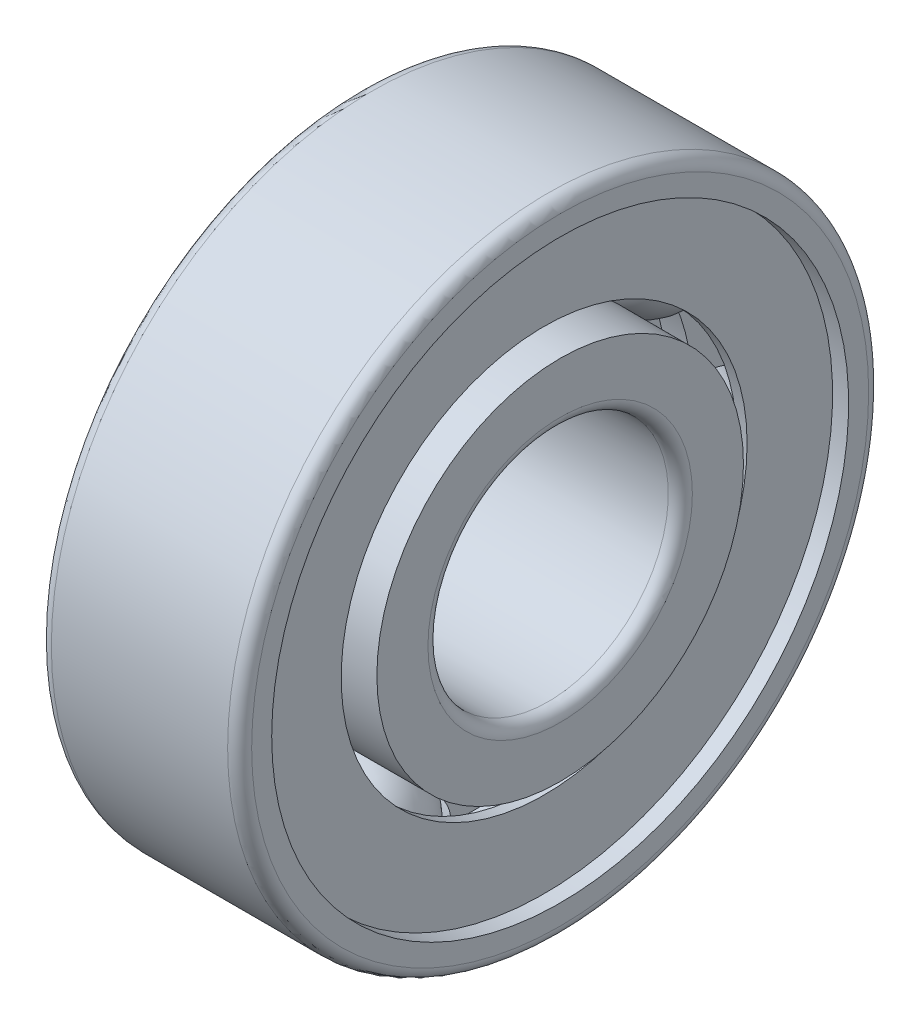
from build123d import *
from build123d.topology import SkipClean

# Parameters (mm, degrees)
SKETCH2_W          = 1.30966
SKETCH2_H          = 1.637075
CIRPATTERN1_COUNT  = 7
SKETCH4_W          = 6.5483
SKETCH4_H          = 3.27415
SKETCH5_W          = 6.5483
SKETCH5_H          = 3.27415
CIRPATTERN2_COUNT  = 7
SKETCH10_W         = 0.535202389
SKETCH10_H         = 3.867755
SKETCH11_R         = 16
CUT_EXTRUDE1_DEPTH = 10


with BuildPart() as part:
    # Sketch2 → Base-Revolve (revolve)
    with BuildSketch(Plane.XY, mode=Mode.PRIVATE) as base_revolve_sk:
        with Locations((0, 11.775)):
            Rectangle(SKETCH2_W, SKETCH2_H)
    revolve(base_revolve_sk.sketch.rotate(Axis((-12.420610377, 0, 0), (1, 0, 0)), 90), axis=Axis((-12.420610377, 0, 0), (1, 0, 0)))

    # Sketch3 → Boss-Revolve1 (revolve)
    with BuildSketch(Plane.XY):
        with BuildLine():
            Line((-3.27415, 11.775), (3.27415, 11.775))
            ThreePointArc((3.27415, 11.775), (0, 8.50085), (-3.27415, 11.775))
        make_face()
    boss_revolve1 = revolve(axis=Axis((-5.568093779, 11.775, 0), (1, 0, 0)))

    # CirPattern1: Boss-Revolve1 ×7 about axis
    cirpattern1_axis = Axis((0, 0, 0), (1, 0, 0))
    for i in range(1, CIRPATTERN1_COUNT):
        add(boss_revolve1.rotate(cirpattern1_axis, i * 360 / CIRPATTERN1_COUNT))

    # Sketch4 → Cut-Revolve1 (revolve, cut)
    with BuildSketch(Plane.XY, mode=Mode.PRIVATE) as cut_revolve1_sk:
        with Locations((0, 14.2306125)):
            Rectangle(SKETCH4_W, SKETCH4_H)
    revolve(cut_revolve1_sk.sketch.rotate(Axis((0, 0, 0), (1, 0, 0)), 66.062644752), axis=Axis((0, 0, 0), (1, 0, 0)), mode=Mode.SUBTRACT)

    # Sketch5 → Cut-Revolve2 (revolve, cut)
    with BuildSketch(Plane.XY, mode=Mode.PRIVATE) as cut_revolve2_sk:
        with Locations((0, 9.3193875)):
            Rectangle(SKETCH5_W, SKETCH5_H)
    revolve(cut_revolve2_sk.sketch.rotate(Axis((0, 0, 0), (1, 0, 0)), 87.161409224), axis=Axis((0, 0, 0), (1, 0, 0)), mode=Mode.SUBTRACT)

    # Sketch6 → Boss-Revolve2 (revolve)
    with BuildSketch(Plane.XY):
        with BuildLine():
            Line((-2.9765, 11.775), (2.9765, 11.775))
            ThreePointArc((2.9765, 11.775), (0, 8.7985), (-2.9765, 11.775))
        make_face()
    boss_revolve2 = revolve(axis=Axis((-5.568093779, 11.775, 0), (1, 0, 0)))

    # CirPattern2: Boss-Revolve2 ×7 about axis
    cirpattern2_axis = Axis((0, 0, 0), (1, 0, 0))
    for i in range(1, CIRPATTERN2_COUNT):
        add(boss_revolve2.rotate(cirpattern2_axis, i * 360 / CIRPATTERN2_COUNT))

    # Sketch7 → Boss-Revolve3 (revolve)
    with BuildSketch(Plane.XY, mode=Mode.PRIVATE) as boss_revolve3_sk:
        with BuildLine():
            Line((-4.4, 16), (4.4, 16))
            ThreePointArc((4.4, 16), (4.824264069, 15.824264069), (5, 15.4))
            Line((5, 15.4), (5, 14.4))
            Line((5, 14.4), (4.2, 14.4))
            Line((4.2, 14.4), (4.2, 14))
            Line((4.2, 14), (3.664797611, 14))
            Line((3.664797611, 14), (3.664797611, 14.4))
            Line((3.664797611, 14.4), (1.381845596, 14.4))
            ThreePointArc((1.381845596, 14.4), (0, 14.7415), (-1.381845596, 14.4))
            Line((-1.381845596, 14.4), (-5, 14.4))
            Line((-5, 14.4), (-5, 15.4))
            ThreePointArc((-5, 15.4), (-4.824264069, 15.824264069), (-4.4, 16))
        make_face()
    revolve(boss_revolve3_sk.sketch.rotate(Axis((0, 0, 0), (1, 0, 0)), 90), axis=Axis((0, 0, 0), (1, 0, 0)))

    # Sketch8 → Boss-Revolve4 (revolve)
    with BuildSketch(Plane.XY, mode=Mode.PRIVATE) as boss_revolve4_sk:
        with BuildLine():
            Line((-5, 9.15), (-1.381845596, 9.15))
            ThreePointArc((-1.381845596, 9.15), (0, 8.8085), (1.381845596, 9.15))
            Line((1.381845596, 9.15), (5, 9.15))
            Line((5, 9.15), (5, 6.6))
            ThreePointArc((5, 6.6), (4.824264069, 6.175735931), (4.4, 6))
            Line((4.4, 6), (-4.4, 6))
            ThreePointArc((-4.4, 6), (-4.824264069, 6.175735931), (-5, 6.6))
            Line((-5, 6.6), (-5, 9.15))
        make_face()
    revolve(boss_revolve4_sk.sketch.rotate(Axis((-12.420610377, 0, 0), (1, 0, 0)), 90), axis=Axis((-12.420610377, 0, 0), (1, 0, 0)))

    # Sketch10 → Boss-Revolve5 (revolve)
    with BuildSketch(Plane.XY, mode=Mode.PRIVATE) as boss_revolve5_sk:
        with Locations((3.932398806, 12.0661225)):
            Rectangle(SKETCH10_W, SKETCH10_H)
    revolve(boss_revolve5_sk.sketch.rotate(Axis((0, 0, 0), (-1, 0, 0)), 257.142857126), axis=Axis((0, 0, 0), (-1, 0, 0)))

    # Sketch11 → Cut-Extrude1 (cut)
    with SkipClean():  # the faces are left unmerged after this step: merging them gives an invalid solid
        with BuildSketch(Plane(origin=(0, 0, 0), x_dir=(0, 0, -1), z_dir=(1, 0, 0))):
            with Locations(Location((0, 0, 0), (0, 0, 180))):
                Circle(SKETCH11_R)
        extrude(amount=-CUT_EXTRUDE1_DEPTH, mode=Mode.SUBTRACT)

    # Mirror All1: part across plane


with BuildPart() as part_1:
    add(part.part)
    add(part.part.mirror(Plane(origin=(0, 0, 0), x_dir=(0, 0, 1), z_dir=(1, 0, 0))))


solid = part_1.part
